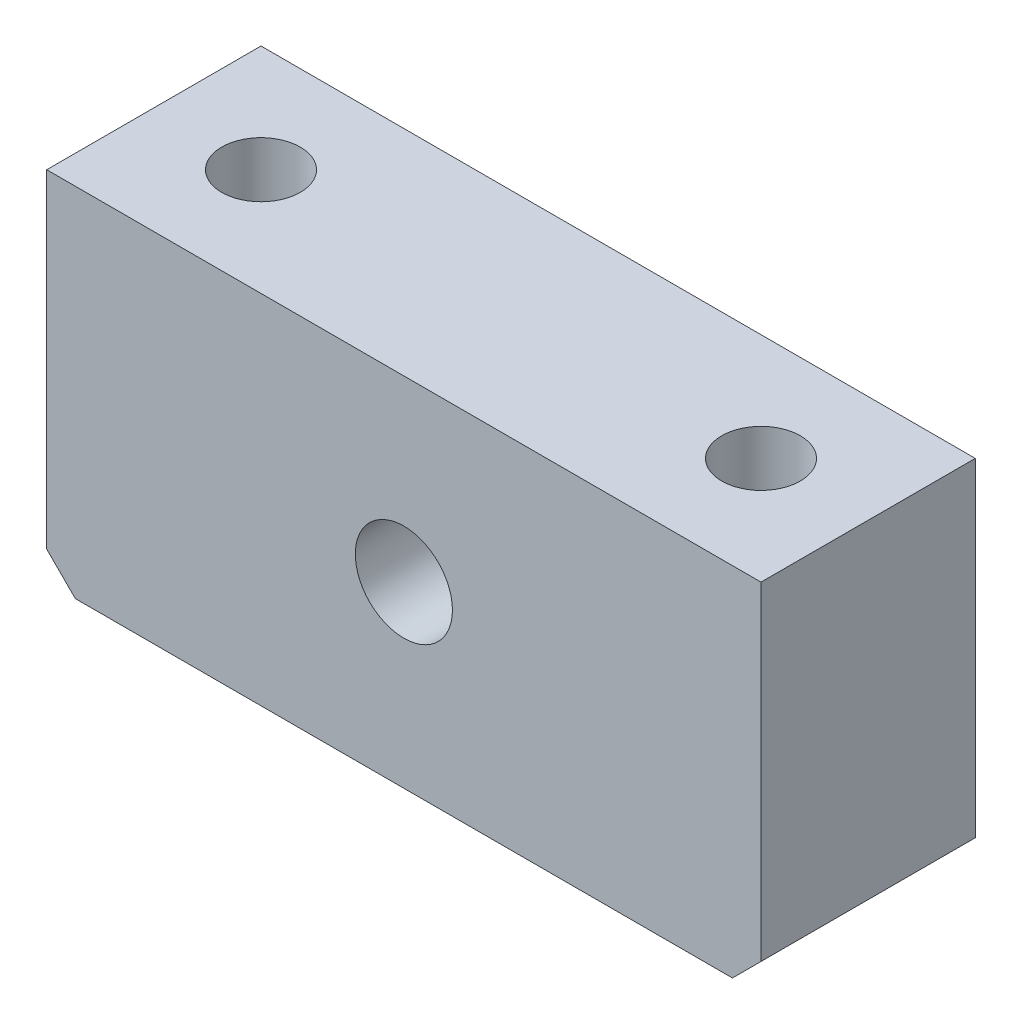
from build123d import *

# Parameters (mm, degrees)
SKETCH_1_W                   = 50
SKETCH_1_H                   = 25
EXTRUDE_1_DEPTH              = 15
CHAMFER_1_SIZE               = 2
HOLE_WIZARD_M5_1_D           = 5.5
HOLE_WIZARD_M5_1_CBORE_D     = 10
HOLE_WIZARD_M5_1_CBORE_DEPTH = 15.7
HOLE_WIZARD_M8_1_D           = 6.8


with BuildPart() as part:
    # 草图1 → 凸台-拉伸1 (new body)
    with BuildSketch(Plane.XY):
        Rectangle(SKETCH_1_W, SKETCH_1_H)
    extrude(amount=EXTRUDE_1_DEPTH)

    # 倒角1
    chamfer_1_edges = [part.edges().sort_by_distance(p)[0] for p in [
        (25, -12.5, 7.5),
        (-25, -12.5, 7.5),
    ]]
    chamfer(chamfer_1_edges, length=CHAMFER_1_SIZE)

    # M5 六角圆柱头螺钉的柱形沉头孔1 (through all)
    with Locations(Plane(origin=(0, -12.5, 0), x_dir=(-1, 0, 0), z_dir=(0, -1, 0))):
        with Locations((-17.5, -7.5), (17.5, -7.5)):
            CounterBoreHole(HOLE_WIZARD_M5_1_D / 2, HOLE_WIZARD_M5_1_CBORE_D / 2, HOLE_WIZARD_M5_1_CBORE_DEPTH)

    # M8 螺纹孔1 (through all)
    with Locations(Plane.XY.offset(15)):
        with Locations((0, 0)):
            Hole(HOLE_WIZARD_M8_1_D / 2)


solid = part.part
